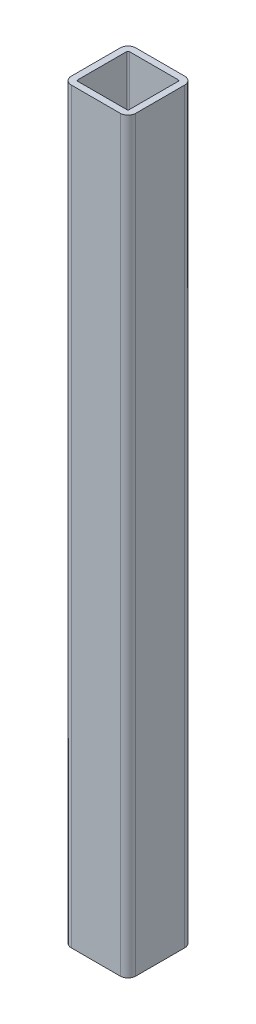
SolidWorks part; units mm, degrees
ref_plane "Front" through (0, 0, 0) normal (0, 0, 1) x (1, 0, 0)
ref_plane "Top" through (0, 0, 0) normal (0, 1, 0) x (1, 0, 0)
ref_plane "Right" through (0, 0, 0) normal (1, 0, 0) x (0, 0, -1)
sketch "草图1" plane through (0, 0, 0) normal (0, 1, 0) x (1, 0, 0)
  line L0 (-19, -7.2781) -> (19, -7.2781)
  line L1 (-19, -12.2781) -> (19, -12.2781)
  line L2 (-25, -6.2781) -> (-25, 31.7219)
  line L3 (-19, 37.7219) -> (19, 37.7219)
  line L4 (25, -6.2781) -> (25, 31.7219)
  line L5 (20, -6.2781) -> (20, 31.7219)
  line L6 (-19, 32.7219) -> (19, 32.7219)
  line L11 (-20, -6.2781) -> (-20, 31.7219)
  arc A0 (-19, -12.2781) -> (-25, -6.2781) centre (-19, -6.2781) cw
  arc A1 (19, -12.2781) -> (25, -6.2781) centre (19, -6.2781) ccw
  arc A2 (19, 37.7219) -> (25, 31.7219) centre (19, 31.7219) cw
  arc A3 (-25, 31.7219) -> (-19, 37.7219) centre (-19, 31.7219) cw
  arc A4 (19, -7.2781) -> (20, -6.2781) centre (19, -6.2781) ccw
  arc A5 (19, 32.7219) -> (20, 31.7219) centre (19, 31.7219) cw
  arc A6 (-20, 31.7219) -> (-19, 32.7219) centre (-19, 31.7219) cw
  arc A7 (-19, -7.2781) -> (-20, -6.2781) centre (-19, -6.2781) cw
  point P9 (25, -12.2781)
  point P12 (25, 37.7219)
  point P15 (-25, 37.7219)
  dimension "D3" = 6
  dimension "D1" = 50
  dimension "D2" = 50
  dimension "D4" = 5
extrude "凸台-拉伸1" add sketch "草图1" along normal blind 580
